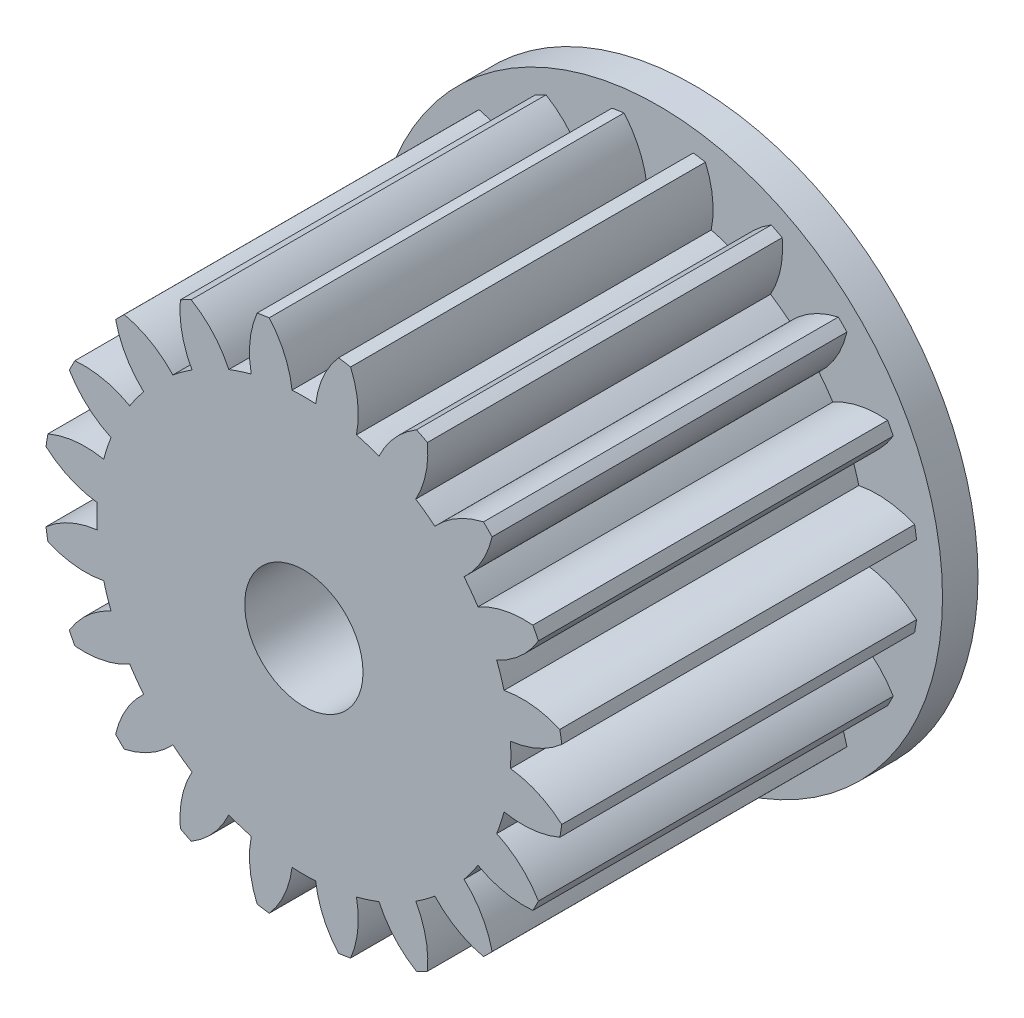
from build123d import *

# Parameters (mm, degrees)
SKETCH1_R           = 12
BOSS_EXTRUDE1_DEPTH = 1.5
BOSS_EXTRUDE2_DEPTH = 15
SKETCH3_R           = 2.5
CUT_EXTRUDE1_DEPTH  = 24
SKETCH4_R           = 7
CUT_EXTRUDE2_DEPTH  = 2


with BuildPart() as part:
    # Sketch1 → Boss-Extrude1 (new body)
    with BuildSketch(Plane.XY):
        Circle(SKETCH1_R)
    extrude(amount=BOSS_EXTRUDE1_DEPTH)

    # Sketch2 → Boss-Extrude2 (add)
    with BuildSketch(Plane.XY.offset(1.5)):
        with BuildLine():
            ThreePointArc((-10.902013697, 1.564204022), (-9.891552344, 0.917308412), (-8.734705318, 0.599171595))
            ThreePointArc((-8.734705318, 0.599171595), (-8.749, 0.099247587), (-8.734705318, -0.40067642))
            ThreePointArc((-8.734705318, -0.40067642), (-9.891552344, -0.718813238), (-10.902013697, -1.365708848))
            ThreePointArc((-10.902013697, -1.365708848), (-10.864571747, -1.621531528), (-10.821127601, -1.876403554))
            ThreePointArc((-10.821127601, -1.876403554), (-9.66022001, -2.179388109), (-8.461683425, -2.124468812))
            ThreePointArc((-8.461683425, -2.124468812), (-8.320793461, -2.604342097), (-8.152713396, -3.075380782))
            ThreePointArc((-8.152713396, -3.075380782), (-9.154630615, -3.735432266), (-9.915734733, -4.662916282))
            ThreePointArc((-9.915734733, -4.662916282), (-9.801071766, -4.89464791), (-9.680994141, -5.123620632))
            ThreePointArc((-9.680994141, -5.123620632), (-8.483278035, -5.053035893), (-7.360373002, -4.630436364))
            ThreePointArc((-7.360373002, -4.630436364), (-7.078089684, -5.043285585), (-6.772677084, -5.4393304))
            ThreePointArc((-6.772677084, -5.4393304), (-7.521589858, -6.376686112), (-7.958834566, -7.493969936))
            ThreePointArc((-7.958834566, -7.493969936), (-7.778174593, -7.678927006), (-7.593217523, -7.859586978))
            ThreePointArc((-7.593217523, -7.859586978), (-6.4759337, -7.422342271), (-5.538577987, -6.673429497))
            ThreePointArc((-5.538577987, -6.673429497), (-5.142533172, -6.978842097), (-4.729683951, -7.261125414))
            ThreePointArc((-4.729683951, -7.261125414), (-5.15228348, -8.384030448), (-5.222868219, -9.581746554))
            ThreePointArc((-5.222868219, -9.581746554), (-4.993895497, -9.701824179), (-4.762163869, -9.816487145))
            ThreePointArc((-4.762163869, -9.816487145), (-3.834679853, -9.055383028), (-3.174628369, -8.053465809))
            ThreePointArc((-3.174628369, -8.053465809), (-2.703589684, -8.221545874), (-2.223716399, -8.362435837))
            ThreePointArc((-2.223716399, -8.362435837), (-2.278635697, -9.560972423), (-1.975651141, -10.721880014))
            ThreePointArc((-1.975651141, -10.721880014), (-1.720779115, -10.765324159), (-1.464956435, -10.802766109))
            ThreePointArc((-1.464956435, -10.802766109), (-0.818060825, -9.792304756), (-0.499924007, -8.63545773))
            ThreePointArc((-0.499924007, -8.63545773), (0, -8.649752413), (0.499924007, -8.63545773))
            ThreePointArc((0.499924007, -8.63545773), (0.818060825, -9.792304756), (1.464956435, -10.802766109))
            ThreePointArc((1.464956435, -10.802766109), (1.720779115, -10.765324159), (1.975651141, -10.721880014))
            ThreePointArc((1.975651141, -10.721880014), (2.278635697, -9.560972423), (2.223716399, -8.362435837))
            ThreePointArc((2.223716399, -8.362435837), (2.703589684, -8.221545874), (3.174628369, -8.053465809))
            ThreePointArc((3.174628369, -8.053465809), (3.834679853, -9.055383028), (4.762163869, -9.816487145))
            ThreePointArc((4.762163869, -9.816487145), (4.993895497, -9.701824179), (5.222868219, -9.581746554))
            ThreePointArc((5.222868219, -9.581746554), (5.15228348, -8.384030448), (4.729683951, -7.261125414))
            ThreePointArc((4.729683951, -7.261125414), (5.142533172, -6.978842097), (5.538577987, -6.673429497))
            ThreePointArc((5.538577987, -6.673429497), (6.4759337, -7.422342271), (7.593217523, -7.859586978))
            ThreePointArc((7.593217523, -7.859586978), (7.778174593, -7.678927006), (7.958834566, -7.493969936))
            ThreePointArc((7.958834566, -7.493969936), (7.521589858, -6.376686112), (6.772677084, -5.4393304))
            ThreePointArc((6.772677084, -5.4393304), (7.078089684, -5.043285585), (7.360373002, -4.630436364))
            ThreePointArc((7.360373002, -4.630436364), (8.483278035, -5.053035893), (9.680994141, -5.123620632))
            ThreePointArc((9.680994141, -5.123620632), (9.801071766, -4.89464791), (9.915734733, -4.662916282))
            ThreePointArc((9.915734733, -4.662916282), (9.154630615, -3.735432266), (8.152713396, -3.075380782))
            ThreePointArc((8.152713396, -3.075380782), (8.320793461, -2.604342097), (8.461683425, -2.124468812))
            ThreePointArc((8.461683425, -2.124468812), (9.66022001, -2.179388109), (10.821127601, -1.876403554))
            ThreePointArc((10.821127601, -1.876403554), (10.864571747, -1.621531528), (10.902013697, -1.365708848))
            ThreePointArc((10.902013697, -1.365708848), (9.891552344, -0.718813238), (8.734705318, -0.40067642))
            ThreePointArc((8.734705318, -0.40067642), (8.749, 0.099247587), (8.734705318, 0.599171595))
            ThreePointArc((8.734705318, 0.599171595), (9.891552344, 0.917308412), (10.902013697, 1.564204022))
            ThreePointArc((10.902013697, 1.564204022), (10.864571747, 1.820026703), (10.821127601, 2.074898729))
            ThreePointArc((10.821127601, 2.074898729), (9.66022001, 2.377883284), (8.461683425, 2.322963986))
            ThreePointArc((8.461683425, 2.322963986), (8.320793461, 2.802837271), (8.152713396, 3.273875956))
            ThreePointArc((8.152713396, 3.273875956), (9.154630615, 3.933927441), (9.915734733, 4.861411456))
            ThreePointArc((9.915734733, 4.861411456), (9.801071766, 5.093143084), (9.680994141, 5.322115806))
            ThreePointArc((9.680994141, 5.322115806), (8.483278035, 5.251531067), (7.360373002, 4.828931538))
            ThreePointArc((7.360373002, 4.828931538), (7.078089684, 5.24178076), (6.772677084, 5.637825574))
            ThreePointArc((6.772677084, 5.637825574), (7.521589858, 6.575181287), (7.958834566, 7.692465111))
            ThreePointArc((7.958834566, 7.692465111), (7.778174593, 7.87742218), (7.593217523, 8.058082153))
            ThreePointArc((7.593217523, 8.058082153), (6.4759337, 7.620837446), (5.538577987, 6.871924671))
            ThreePointArc((5.538577987, 6.871924671), (5.142533172, 7.177337271), (4.729683951, 7.459620589))
            ThreePointArc((4.729683951, 7.459620589), (5.15228348, 8.582525623), (5.222868219, 9.780241729))
            ThreePointArc((5.222868219, 9.780241729), (4.993895497, 9.900319353), (4.762163869, 10.01498232))
            ThreePointArc((4.762163869, 10.01498232), (3.834679853, 9.253878203), (3.174628369, 8.251960983))
            ThreePointArc((3.174628369, 8.251960983), (2.703589684, 8.420041048), (2.223716399, 8.560931012))
            ThreePointArc((2.223716399, 8.560931012), (2.278635697, 9.759467597), (1.975651141, 10.920375189))
            ThreePointArc((1.975651141, 10.920375189), (1.720779115, 10.963819334), (1.464956435, 11.001261284))
            ThreePointArc((1.464956435, 11.001261284), (0.818060825, 9.990799931), (0.499924007, 8.833952905))
            ThreePointArc((0.499924007, 8.833952905), (0, 8.848247587), (-0.499924007, 8.833952905))
            ThreePointArc((-0.499924007, 8.833952905), (-0.818060825, 9.990799931), (-1.464956435, 11.001261284))
            ThreePointArc((-1.464956435, 11.001261284), (-1.720779115, 10.963819334), (-1.975651141, 10.920375189))
            ThreePointArc((-1.975651141, 10.920375189), (-2.278635697, 9.759467597), (-2.223716399, 8.560931012))
            ThreePointArc((-2.223716399, 8.560931012), (-2.703589684, 8.420041048), (-3.174628369, 8.251960983))
            ThreePointArc((-3.174628369, 8.251960983), (-3.834679853, 9.253878203), (-4.762163869, 10.01498232))
            ThreePointArc((-4.762163869, 10.01498232), (-4.993895497, 9.900319353), (-5.222868219, 9.780241729))
            ThreePointArc((-5.222868219, 9.780241729), (-5.15228348, 8.582525623), (-4.729683951, 7.459620589))
            ThreePointArc((-4.729683951, 7.459620589), (-5.142533172, 7.177337271), (-5.538577987, 6.871924671))
            ThreePointArc((-5.538577987, 6.871924671), (-6.4759337, 7.620837446), (-7.593217523, 8.058082153))
            ThreePointArc((-7.593217523, 8.058082153), (-7.778174593, 7.87742218), (-7.958834566, 7.692465111))
            ThreePointArc((-7.958834566, 7.692465111), (-7.521589858, 6.575181287), (-6.772677084, 5.637825574))
            ThreePointArc((-6.772677084, 5.637825574), (-7.078089684, 5.24178076), (-7.360373002, 4.828931538))
            ThreePointArc((-7.360373002, 4.828931538), (-8.483278035, 5.251531067), (-9.680994141, 5.322115806))
            ThreePointArc((-9.680994141, 5.322115806), (-9.801071766, 5.093143084), (-9.915734733, 4.861411456))
            ThreePointArc((-9.915734733, 4.861411456), (-9.154630615, 3.933927441), (-8.152713396, 3.273875956))
            ThreePointArc((-8.152713396, 3.273875956), (-8.320793461, 2.802837271), (-8.461683425, 2.322963986))
            ThreePointArc((-8.461683425, 2.322963986), (-9.66022001, 2.377883284), (-10.821127601, 2.074898729))
            ThreePointArc((-10.821127601, 2.074898729), (-10.864571747, 1.820026703), (-10.902013697, 1.564204022))
        make_face()
    extrude(amount=BOSS_EXTRUDE2_DEPTH)

    # Sketch3 → Cut-Extrude1 (cut)
    with BuildSketch(Plane.XY.offset(16.5)):
        Circle(SKETCH3_R)
    extrude(amount=-CUT_EXTRUDE1_DEPTH, mode=Mode.SUBTRACT)

    # Sketch4 → Cut-Extrude2 (cut)
    with BuildSketch(Plane(origin=(0, 0, 0), x_dir=(-1, 0, 0), z_dir=(0, 0, -1))):
        Circle(SKETCH4_R)
    extrude(amount=-CUT_EXTRUDE2_DEPTH, mode=Mode.SUBTRACT)


solid = part.part
